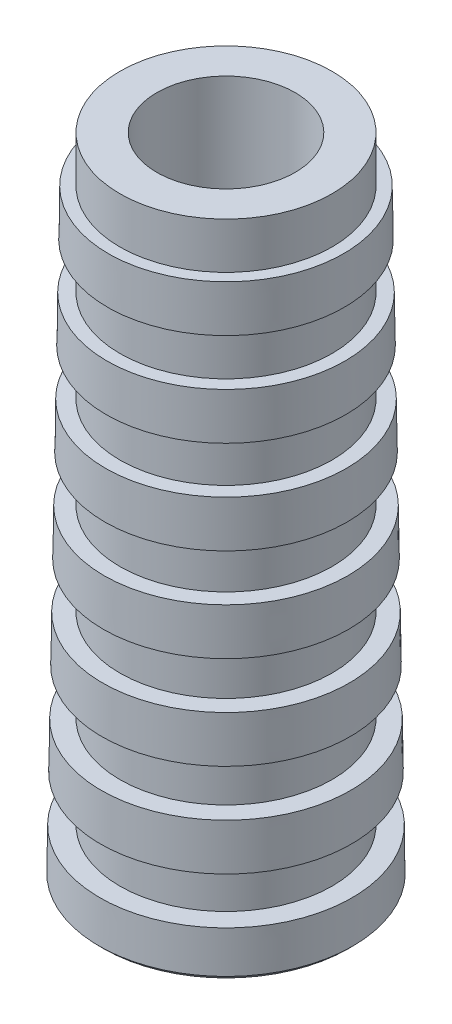
SolidWorks part; units mm, degrees
ref_plane "前视基准面" through (0, 0, 0) normal (0, 0, 1) x (1, 0, 0)
ref_plane "上视基准面" through (0, 0, 0) normal (0, 1, 0) x (1, 0, 0)
ref_plane "右视基准面" through (0, 0, 0) normal (1, 0, 0) x (0, 0, -1)
ref_plane "基准面4" through (0, 0, 0) normal (0, 0, -1) x (-1, 0, 0)
sketch "草图1" plane through (0, 0, 0) normal (0, 0, -1) x (-1, 0, 0)
  line L0 (-23, -215) -> (-26.4222, -215)
  line L1 (-26.4222, -215) -> (-26.5762, -225)
  line L2 (-26.5762, -225) -> (-23, -225)
  line L3 (-23, -225) -> (-23, -235)
  line L4 (-23, -235) -> (-26.7302, -235)
  line L5 (-26.7302, -235) -> (-26.8841, -245)
  line L6 (-26.8841, -245) -> (-23, -245)
  line L7 (-23, -245) -> (-23, -255)
  line L8 (-23, -255) -> (-27.0381, -255)
  line L9 (-27.0381, -255) -> (-27.1921, -265)
  line L10 (-27.1921, -265) -> (-23, -265)
  line L11 (-23, -265) -> (-23, -275)
  line L12 (-23, -275) -> (-27.346, -275)
  line L13 (-27.346, -275) -> (-27.4848, -284.0152)
  line L14 (-27.4848, -284.0152) -> (-26.5, -285)
  line L15 (-26.5, -285) -> (-16, -285)
  line L16 (-16, -285) -> (-15, -284)
  line L17 (-15, -284) -> (-15, -145)
  line L18 (-15, -145) -> (-23, -145)
  line L19 (-23, -145) -> (-23, -155)
  line L20 (-23, -155) -> (-25.4984, -155)
  line L21 (-25.4984, -155) -> (-25.6524, -165)
  line L22 (-25.6524, -165) -> (-23, -165)
  line L23 (-23, -165) -> (-23, -175)
  line L24 (-23, -175) -> (-25.8064, -175)
  line L25 (-25.8064, -175) -> (-25.9603, -185)
  line L26 (-25.9603, -185) -> (-23, -185)
  line L27 (-23, -185) -> (-23, -195)
  line L28 (-23, -195) -> (-26.1143, -195)
  line L29 (-26.1143, -195) -> (-26.2683, -205)
  line L30 (-26.2683, -205) -> (-23, -205)
  line L31 (-23, -205) -> (-23, -215)
  line L32 (0, -285) -> (0, -145) construction
revolve "旋转1" add sketch "草图1" angle 360 about L32
